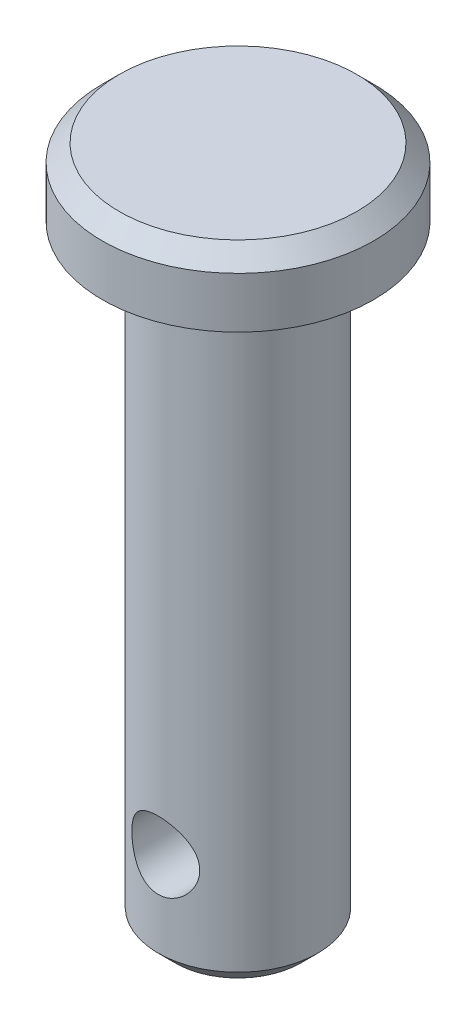
SolidWorks part; units mm, degrees
material "Plain Carbon Steel"
ref_plane "Front Plane" through (0, 0, 0) normal (0, 0, 1) x (1, 0, 0)
ref_plane "Top Plane" through (0, 0, 0) normal (0, 1, 0) x (1, 0, 0)
ref_plane "Right Plane" through (0, 0, 0) normal (1, 0, 0) x (0, 0, -1)
sketch "Sketch1" plane through (0, 0, 0) normal (0, 0, 1) x (1, 0, 0)
  line L0 (0, -273.1339) -> (0, 13383.5599) construction
  line L1 (0, 0) -> (4, 0)
  line L2 (4, 0) -> (4, -2)
  line L3 (4, -2) -> (2.35, -2)
  line L4 (2.35, -2) -> (2.35, -20)
  line L5 (2.35, -20) -> (0, -20)
  line L6 (0, 0) -> (0, -20)
  dimension "D1" = 4
  dimension "D2" = 2.35
  dimension "D3" = 2
  dimension "D4" = 20
revolve "Revolve1" add sketch "Sketch1" angle 360 about L0
fillet "Fillet1" radius 0.5 1 edges at (2.35, -2, 0)
chamfer "Chamfer1" distance 0.5 angle 45 2 edges at (2.35, -20, 0) (4, 0, 0)
sketch "Sketch2" plane through (0, 0, 0) normal (0, 0, 1) x (1, 0, 0)
  line L0 (0, -1000) -> (0, 49000) construction
  line L1 (-4, -2) -> (4, -2) construction
  circle A0 centre (0, -17) radius 1
  dimension "D2" = 2
  dimension "D1" = 15
extrude "Cut-Extrude1" cut sketch "Sketch2" against normal through all both and the other way through all
